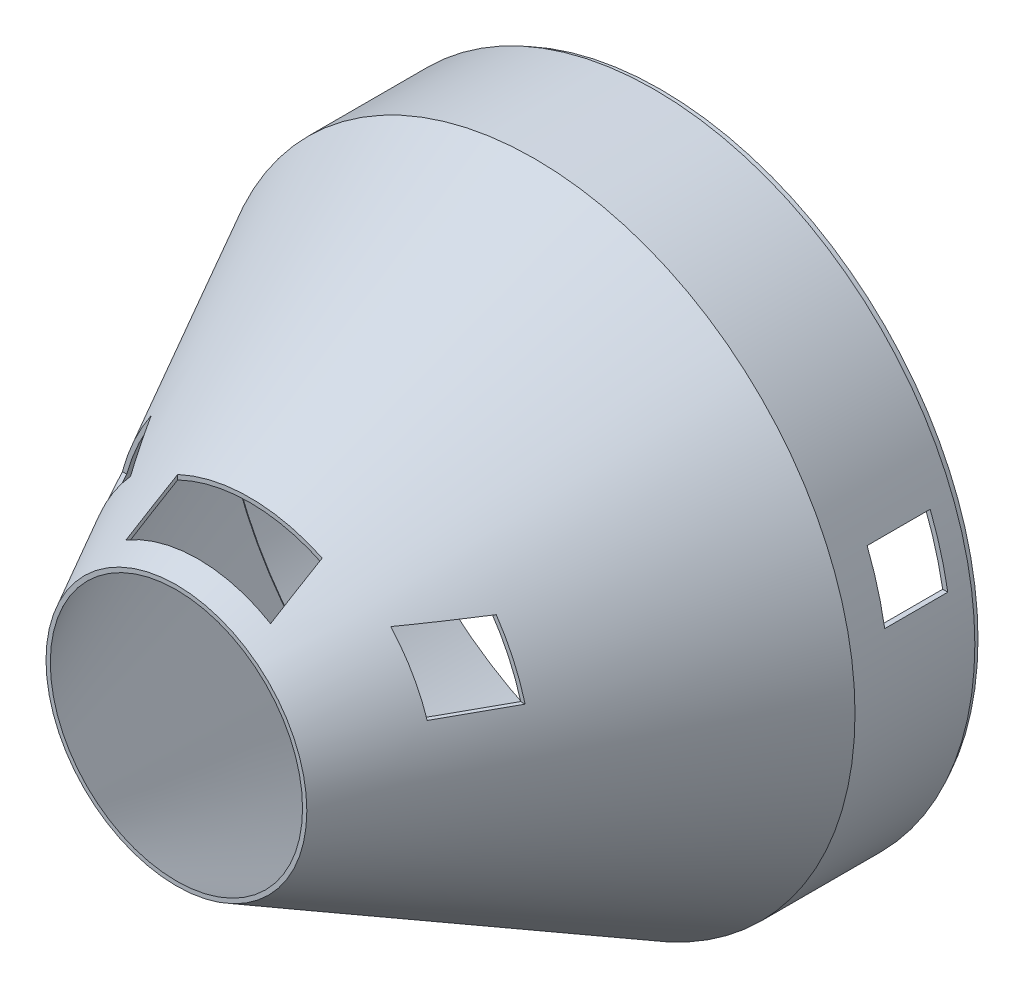
from build123d import *

# Parameters (mm, degrees)
SKETCH2_R           = 254
SKETCH2_R_2         = 250
BOSS_EXTRUDE1_DEPTH = 100
SKETCH7_W           = 50
SKETCH7_H           = 50
CUT_EXTRUDE3_DEPTH  = 500
SKETCH8_R           = 254
SKETCH8_R_2         = 251.5
CUT_EXTRUDE4_DEPTH  = 5
CUT_EXTRUDE5_START  = 100
SKETCH9_W           = 114.623557318
SKETCH9_H           = 40.936984757
CUT_EXTRUDE5_DEPTH  = 200


with BuildPart() as part:
    # Sketch2 → Boss-Extrude1 (new body)
    with BuildSketch(Plane.XY):
        Circle(SKETCH2_R)
        Circle(SKETCH2_R_2, mode=Mode.SUBTRACT)
    extrude(amount=BOSS_EXTRUDE1_DEPTH)

    # Sketch5 → Revolve1 (revolve)
    with BuildSketch(Plane(origin=(0, 0, 0), x_dir=(1, 0, 0), z_dir=(0, 1, 0)), mode=Mode.PRIVATE) as revolve1_sk:
        Polygon((254, -100), (103.395722574, -384), (100, -384), (250.604277426, -100), align=None)
    revolve(revolve1_sk.sketch.rotate(Axis((0, 0, 0), (0, 0, 1)), 180), axis=Axis((0, 0, 0), (0, 0, 1)))

    # Sketch7 → Cut-Extrude3 (cut, symmetric)
    with BuildSketch(Plane(origin=(0, 0, 0), x_dir=(0, 0, -1), z_dir=(1, 0, 0))):
        with Locations((-47.8, 67.9)):
            Rectangle(SKETCH7_W, SKETCH7_H)
        with Locations((-292.2, 67.9)):
            Rectangle(SKETCH7_W, SKETCH7_H)
    extrude(amount=CUT_EXTRUDE3_DEPTH, both=True, mode=Mode.SUBTRACT)

    # Sketch8 → Cut-Extrude4 (cut)
    with BuildSketch(Plane(origin=(0, 0, 0), x_dir=(-1, 0, 0), z_dir=(0, 0, -1))):
        Circle(SKETCH8_R)
        Circle(SKETCH8_R_2, mode=Mode.SUBTRACT)
    extrude(amount=-CUT_EXTRUDE4_DEPTH, mode=Mode.SUBTRACT)

    # Sketch9 → Cut-Extrude5 (cut)
    with BuildSketch(Plane(origin=(600, 66.233541641, 45.300312461), x_dir=(1, 0, 0), z_dir=(0, 1, 0)).offset(CUT_EXTRUDE5_START)):
        with Locations((-599.905010531, -300.978332918)):
            Rectangle(SKETCH9_W, SKETCH9_H)
    extrude(amount=-CUT_EXTRUDE5_DEPTH, mode=Mode.SUBTRACT)


solid = part.part
